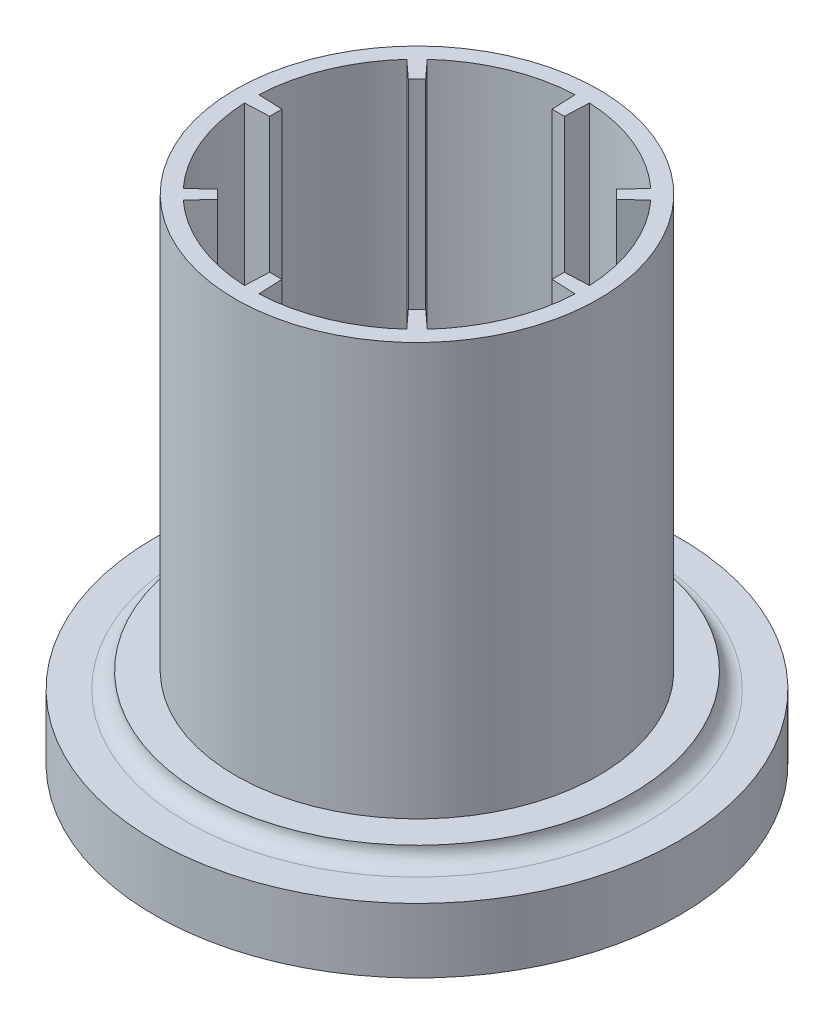
SolidWorks part; units mm, degrees
ref_plane "前视基准面" through (0, 0, 0) normal (0, 0, 1) x (1, 0, 0)
ref_plane "上视基准面" through (0, 0, 0) normal (0, 1, 0) x (1, 0, 0)
ref_plane "右视基准面" through (0, 0, 0) normal (1, 0, 0) x (0, 0, -1)
sketch "草图1" plane through (0, 0, 0) normal (0, 0, 1) x (1, 0, 0)
  line L0 (0, 407.8626) -> (0, -474.5572) construction
  line L1 (-325, 31.7752) -> (-205, 31.7752)
  line L2 (-325, 31.7752) -> (-325, 111.7752)
  line L3 (-325, 111.7752) -> (-285, 111.7752)
  line L5 (-265, 131.7752) -> (-225, 131.7752)
  line L6 (-225, 131.7752) -> (-225, 443.7952)
  line L7 (-225, 443.7952) -> (-205, 443.7952)
  line L8 (-205, 443.7952) -> (-205, 393.7952)
  line L9 (-205, 393.7952) -> (-140, 393.7952)
  line L10 (-105, 388.7952) -> (-105, 363.7952)
  line L11 (-105, 363.7952) -> (-205, 363.7952)
  line L12 (-205, 363.7952) -> (-205, 151.7752)
  line L13 (-205, 151.7752) -> (-125, 151.7752)
  line L14 (-125, 151.7752) -> (-125, 101.7752)
  line L15 (-125, 101.7752) -> (-145, 101.7752)
  line L16 (-145, 101.7752) -> (-145, 121.7752)
  line L17 (-155, 131.7752) -> (-195, 131.7752)
  line L18 (-205, 121.7752) -> (-205, 31.7752)
  line L19 (-140, 393.7952) -> (-140, 388.7952)
  line L20 (-140, 388.7952) -> (-105, 388.7952)
  arc A0 (-285, 111.7752) -> (-265, 131.7752) centre (-285, 131.7752) ccw
  arc A1 (-145, 121.7752) -> (-155, 131.7752) centre (-155, 121.7752) ccw
  arc A2 (-205, 121.7752) -> (-195, 131.7752) centre (-195, 121.7752) cw
  dimension "D17" = 10
  dimension "D1" = 205
  dimension "D3" = 80
  dimension "D4" = 50
  dimension "D5" = 20
  dimension "D6" = 20
  dimension "D7" = 205
  dimension "D8" = 100
  dimension "D9" = 30
  dimension "D10" = 65
  dimension "D11" = 205
  dimension "D12" = 25
  dimension "D13" = 50
  dimension "D14" = 20
  dimension "D15" = 40
  dimension "D16" = 80
  dimension "D18" = 312.02
  dimension "D19" = 100
  dimension "D20" = 20
revolve "旋转1" add sketch "草图1" angle 360 about L0
sketch "草图3" plane through (0, 0, 0) normal (0, 0, 1) x (1, 0, 0)
  line L0 (-205, 443.7952) -> (-140, 393.7952)
  line L1 (-140, 393.7952) -> (-205, 393.7952)
  line L2 (-205, 393.7952) -> (-205, 443.7952)
  line L3 (-105, 363.7952) -> (-163.0309, 295.8048)
  line L4 (-205, 363.7952) -> (-205, 136.565)
  line L5 (-155, 136.565) -> (-173.9233, 136.565)
  line L6 (-205, 136.565) -> (-173.9233, 136.565)
  line L7 (-175, 178.9643) -> (-175, 263.3449)
  line L8 (-145, 101.7752) -> (-165, 101.7752)
  line L10 (-165, 101.7752) -> (-205, 31.7752)
  line L11 (-205, 121.7752) -> (-205, 31.7752)
  line L12 (-155, 131.7752) -> (-195, 131.7752)
  line L14 (-145, 101.7752) -> (-145, 121.7752)
  line L16 (-205, 363.7952) -> (-105, 363.7952)
  arc A0 (-163.0309, 295.8048) -> (-175, 263.3449) centre (-125, 263.3449) ccw
  arc A2 (-205, 121.7752) -> (-195, 131.7752) centre (-195, 121.7752) cw
  arc A3 (-145, 121.7752) -> (-155, 131.7752) centre (-155, 121.7752) ccw
  spline S0 degree 2 poles (-175, 178.9643) (-175.0714, 153.1548) (-155, 136.565) knots 0 0 0 1 1 1
  dimension "D1" = 50
revolve "旋转2" add sketch "草图3" angle 5 mid plane about L0
pattern_circular "阵列(圆周)1" count 8 over 360 of "旋转2"
sketch "草图4" plane through (0, 388.7952, 0) normal (0, 1, 0) x (1, 0, 0)
  circle A0 centre (115, 0) radius 5
  circle A1 centre (81.3173, -81.3173) radius 5
  circle A2 centre (0, -115) radius 5
  circle A3 centre (-81.3173, -81.3173) radius 5
  circle A4 centre (-115, 0) radius 5
  circle A5 centre (-81.3173, 81.3173) radius 5
  circle A6 centre (0, 115) radius 5
  circle A7 centre (81.3173, 81.3173) radius 5
  point P19 (0, 0)
  dimension "D1" = 10
  dimension "D2" = 115
  dimension "D3" = 8
extrude "切除-拉伸1" cut sketch "草图4" against normal up to next
sketch "草图5" plane through (0, 0, 0) normal (1, 0, 0) x (0, 0, -1)
  line L0 (0, 483.7281) -> (0, -762.2293) construction
ref_plane "基准面1" through (0, 0, 0) normal (-0.3827, 0, 0.9239) x (0, -1, 0)
sketch "草图6" plane through (0, 0, 0) normal (-0.3827, 0, 0.9239) x (0, -1, 0)
  line L0 (-483.7281, 0) -> (762.2293, 0) construction
  line L1 (-131.7752, 265) -> (-131.7752, -62.12) construction
  line L2 (-131.7752, 265) -> (-131.7752, -265) construction
  line L3 (-131.7752, 225) -> (-131.7752, -225) construction
  circle A1 centre (-371.7752, 0) radius 10
  circle A2 centre (-251.7752, 0) radius 10
  dimension "D2" = 120
  dimension "D3" = 120
extrude "切除-拉伸2" cut sketch "草图6" against normal blind 260
sketch "草图7" plane through (0, 443.7952, 0) normal (0, 1, 0) x (1, 0, 0)
  circle A0 centre (0, 0) radius 225 construction
  circle A1 centre (0, 0) radius 225
extrude "切除-拉伸3" cut sketch "草图7" against normal up to vertex
sketch "草图8" plane through (0, 263.3449, 0) normal (0, 1, 0) x (1, 0, 0)
  line L16 (-204.8049, 8.942) -> (-174.8334, 7.6334)
  line L17 (-129.0235, 118.2283) -> (-151.1419, 138.496)
  line L18 (-138.496, 151.1419) -> (-118.2283, 129.0235)
  line L19 (-7.6334, 174.8334) -> (-8.942, 204.8049)
  line L20 (8.942, 204.8049) -> (7.6334, 174.8334)
  line L21 (118.2283, 129.0235) -> (138.496, 151.1419)
  line L22 (151.1419, 138.496) -> (129.0235, 118.2283)
  line L23 (174.8334, 7.6334) -> (204.8049, 8.942)
  line L24 (204.8049, -8.942) -> (174.8334, -7.6334)
  line L25 (129.0235, -118.2283) -> (151.1419, -138.496)
  line L26 (138.496, -151.1419) -> (118.2283, -129.0235)
  line L27 (7.6334, -174.8334) -> (8.942, -204.8049)
  line L28 (-8.942, -204.8049) -> (-7.6334, -174.8334)
  line L29 (-118.2283, -129.0235) -> (-138.496, -151.1419)
  line L30 (-151.1419, -138.496) -> (-129.0235, -118.2283)
  line L31 (-174.8334, -7.6334) -> (-204.8049, -8.942)
  line L32 (-204.8049, 8.942) -> (-174.8334, 7.6334)
  line L33 (-129.0235, 118.2283) -> (-151.1419, 138.496)
  line L34 (-138.496, 151.1419) -> (-118.2283, 129.0235)
  line L35 (-7.6334, 174.8334) -> (-8.942, 204.8049)
  line L36 (8.942, 204.8049) -> (7.6334, 174.8334)
  line L37 (118.2283, 129.0235) -> (138.496, 151.1419)
  line L38 (151.1419, 138.496) -> (129.0235, 118.2283)
  line L39 (174.8334, 7.6334) -> (204.8049, 8.942)
  line L40 (204.8049, -8.942) -> (174.8334, -7.6334)
  line L41 (129.0235, -118.2283) -> (151.1419, -138.496)
  line L42 (138.496, -151.1419) -> (118.2283, -129.0235)
  line L43 (7.6334, -174.8334) -> (8.942, -204.8049)
  line L44 (-8.942, -204.8049) -> (-7.6334, -174.8334)
  line L45 (-118.2283, -129.0235) -> (-138.496, -151.1419)
  line L46 (-151.1419, -138.496) -> (-129.0235, -118.2283)
  line L47 (-174.8334, -7.6334) -> (-204.8049, -8.942)
  circle A0 centre (0, 0) radius 225 construction
  circle A1 centre (0, 0) radius 225
  arc A16 (-151.1419, 138.496) -> (-204.8049, 8.942) centre (0, 0) ccw
  arc A17 (-118.2283, 129.0235) -> (-129.0235, 118.2283) centre (0, 0) ccw
  arc A18 (-8.942, 204.8049) -> (-138.496, 151.1419) centre (0, 0) ccw
  arc A19 (7.6334, 174.8334) -> (-7.6334, 174.8334) centre (0, 0) ccw
  arc A20 (138.496, 151.1419) -> (8.942, 204.8049) centre (0, 0) ccw
  arc A21 (129.0235, 118.2283) -> (118.2283, 129.0235) centre (0, 0) ccw
  arc A22 (204.8049, 8.942) -> (151.1419, 138.496) centre (0, 0) ccw
  arc A23 (174.8334, -7.6334) -> (174.8334, 7.6334) centre (0, 0) ccw
  arc A24 (151.1419, -138.496) -> (204.8049, -8.942) centre (0, 0) ccw
  arc A25 (118.2283, -129.0235) -> (129.0235, -118.2283) centre (0, 0) ccw
  arc A26 (8.942, -204.8049) -> (138.496, -151.1419) centre (0, 0) ccw
  arc A27 (-7.6334, -174.8334) -> (7.6334, -174.8334) centre (0, 0) ccw
  arc A28 (-138.496, -151.1419) -> (-8.942, -204.8049) centre (0, 0) ccw
  arc A29 (-129.0235, -118.2283) -> (-118.2283, -129.0235) centre (0, 0) ccw
  arc A30 (-204.8049, -8.942) -> (-151.1419, -138.496) centre (0, 0) ccw
  arc A31 (-174.8334, 7.6334) -> (-174.8334, -7.6334) centre (0, 0) ccw
  arc A32 (-151.1419, 138.496) -> (-204.8049, 8.942) centre (0, 0) ccw
  arc A33 (-118.2283, 129.0235) -> (-129.0235, 118.2283) centre (0, 0) ccw
  arc A34 (-8.942, 204.8049) -> (-138.496, 151.1419) centre (0, 0) ccw
  arc A35 (7.6334, 174.8334) -> (-7.6334, 174.8334) centre (0, 0) ccw
  arc A36 (138.496, 151.1419) -> (8.942, 204.8049) centre (0, 0) ccw
  arc A37 (129.0235, 118.2283) -> (118.2283, 129.0235) centre (0, 0) ccw
  arc A38 (204.8049, 8.942) -> (151.1419, 138.496) centre (0, 0) ccw
  arc A39 (174.8334, -7.6334) -> (174.8334, 7.6334) centre (0, 0) ccw
  arc A40 (151.1419, -138.496) -> (204.8049, -8.942) centre (0, 0) ccw
  arc A41 (118.2283, -129.0235) -> (129.0235, -118.2283) centre (0, 0) ccw
  arc A42 (8.942, -204.8049) -> (138.496, -151.1419) centre (0, 0) ccw
  arc A43 (-7.6334, -174.8334) -> (7.6334, -174.8334) centre (0, 0) ccw
  arc A44 (-138.496, -151.1419) -> (-8.942, -204.8049) centre (0, 0) ccw
  arc A45 (-129.0235, -118.2283) -> (-118.2283, -129.0235) centre (0, 0) ccw
  arc A46 (-204.8049, -8.942) -> (-151.1419, -138.496) centre (0, 0) ccw
  arc A47 (-174.8334, 7.6334) -> (-174.8334, -7.6334) centre (0, 0) ccw
  dimension "D1" = 0
extrude "凸台-拉伸1" add sketch "草图8" along normal blind 379.63
